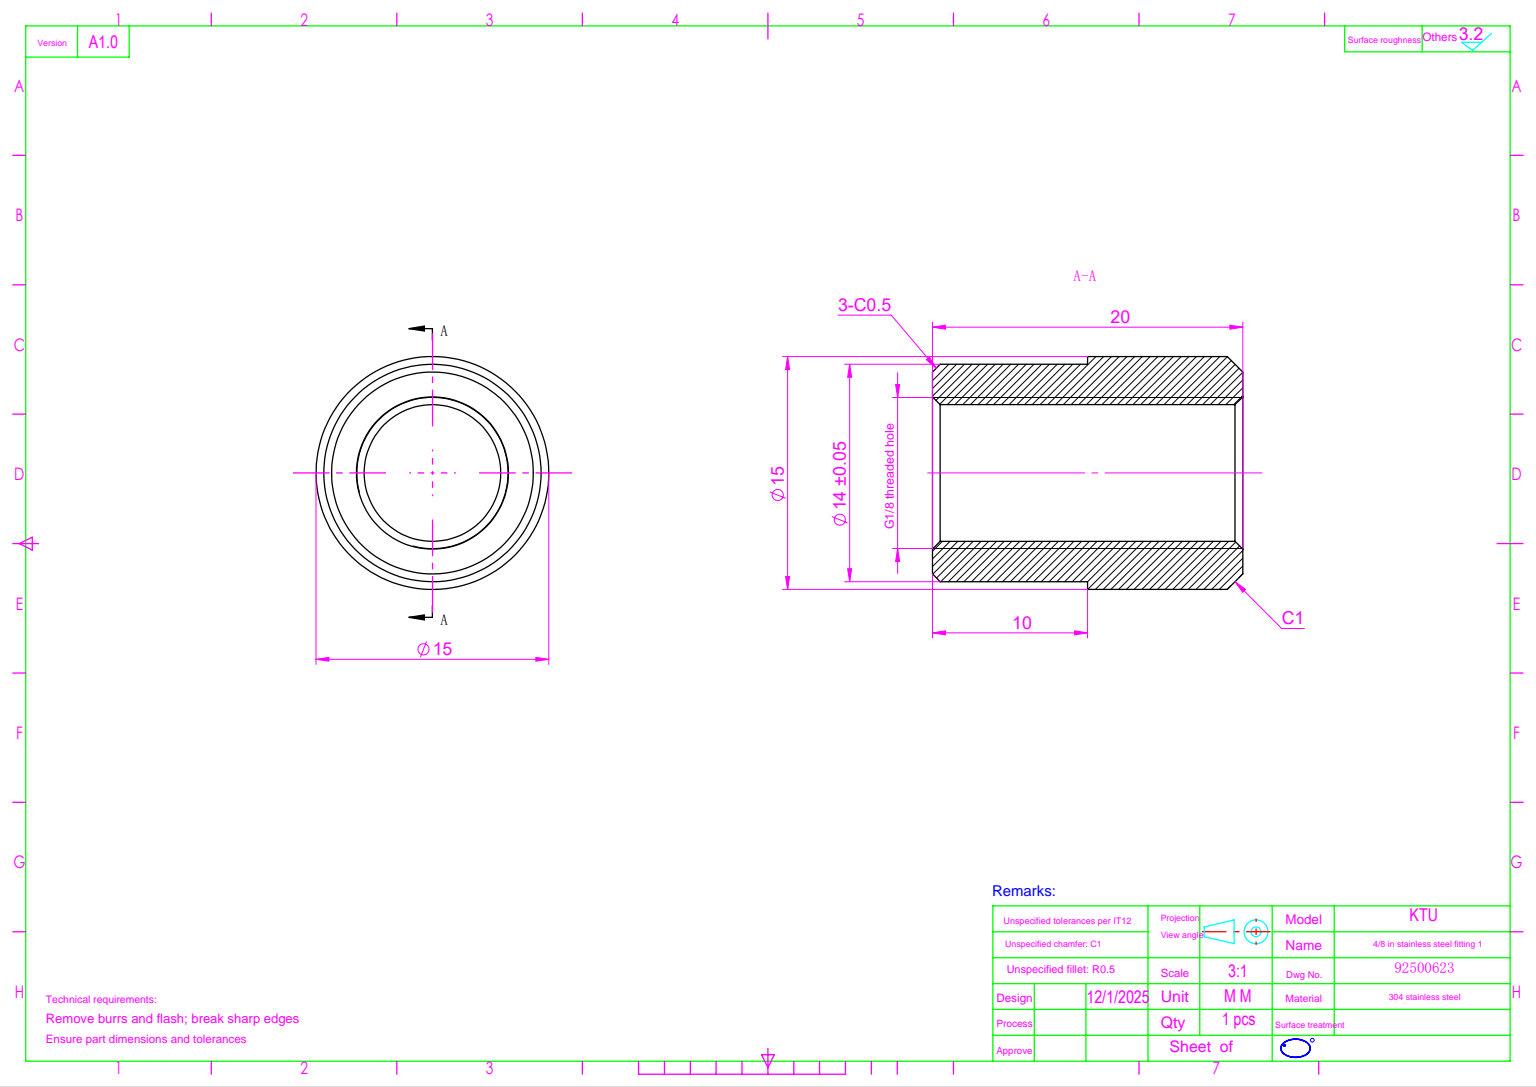
SolidWorks part; units mm, degrees
ref_plane "前视基准面" through (0, 0, 0) normal (0, 0, 1) x (1, 0, 0)
ref_plane "上视基准面" through (0, 0, 0) normal (0, 1, 0) x (1, 0, 0)
ref_plane "右视基准面" through (0, 0, 0) normal (1, 0, 0) x (0, 0, -1)
sketch "草图1" plane through (0, 0, 0) normal (0, 0, 1) x (1, 0, 0)
  circle A0 centre (0, 0) radius 7.5
  dimension "D1" = 15
extrude "凸台-拉伸1" add sketch "草图1" along normal blind 20
sketch "草图2" plane through (0, 0, 20) normal (0, 0, 1) x (1, 0, 0)
  circle A0 centre (0, 0) radius 7
  dimension "D1" = 14
extrude "切除-拉伸1" cut sketch "草图2" against normal blind 10 flip side to cut
hole_wizard "G1/8 螺纹孔1" positions "草图3" profile "草图4" tap size "G1/8" standard "GB" end condition through all
sketch "草图3" plane through (0, 0, 20) normal (0, 0, 1) x (1, 0, 0)
  point P0 (0, 0)
cosmetic thread "孔螺蚊线1" parameters "D2"=9.728
sketch "草图4" plane through (0, 0, 20) normal (1, 0, 0) x (0, -1, 0)
  line L0 (0, 0) -> (0, 20)
  line L1 (0, 20) -> (4.4, 20)
  line L2 (4.4, 20) -> (4.4, 0)
  line L5 (4.4, 0) -> (0, 0)
  line L11 (0, -6.35) -> (0, 107.95) construction
  dimension "通孔螺纹孔钻头直径" = 8.8
  dimension "通孔螺纹孔钻头深度" = 20
sketch "草图5" plane through (0, 0, 0) normal (0, 1, 0) x (1, 0, 0)
  line L0 (7.5, 0) -> (-7.5, 0) construction
  circle A0 centre (0, -5) radius 3
  dimension "D1" = 6
  dimension "D2" = 5
extrude "切除-拉伸2" [suppressed] cut sketch "草图5" against normal through all
chamfer "倒角1" distance 1 angle 45 1 edges at (7.5, 0, 0)
chamfer "倒角2" distance 0.5 angle 45 3 edges at (4.4, 0, 20) (7, 0, 20) (4.4, 0, 0)
